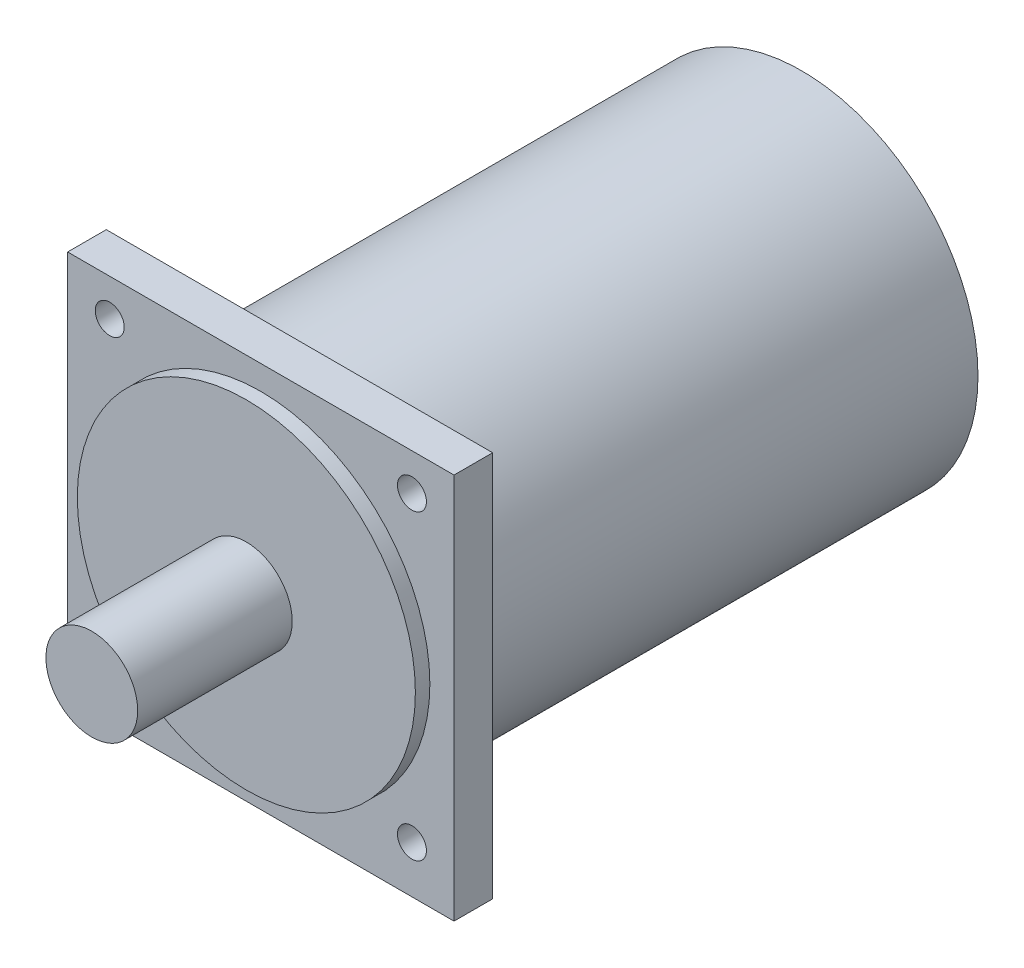
SolidWorks part; units mm, degrees
ref_plane "前视" through (0, 0, 0) normal (0, 0, 1) x (1, 0, 0)
ref_plane "上视" through (0, 0, 0) normal (0, 1, 0) x (1, 0, 0)
ref_plane "右视" through (0, 0, 0) normal (1, 0, 0) x (0, 0, -1)
sketch "草图1" plane through (0, 0, 0) normal (0, 0, 1) x (1, 0, 0)
  line L1 (0, 0) -> (80, 0)
  line L2 (0, 0) -> (0, 80)
  line L3 (0, 80) -> (80, 80)
  line L4 (80, 0) -> (80, 80)
  dimension "D1" = 80
  dimension "D2" = 80
extrude "拉伸1" add sketch "草图1" along normal blind 8
sketch "草图2" plane through (0, 0, 8) normal (0, 0, 1) x (1, 0, 0)
  line L0 (0, 40) -> (80, 40) construction
  line L1 (0, 80) -> (0, 0) construction
  line L2 (80, 0) -> (80, 80) construction
  circle A0 centre (40, 40) radius 35
  dimension "D1" = 70
extrude "拉伸2" add sketch "草图2" along normal blind 3
sketch "草图3" plane through (0, 0, 11) normal (0, 0, 1) x (1, 0, 0)
  circle A0 centre (40, 40) radius 9.5
  circle A1 centre (40, 40) radius 35 construction
  dimension "D1" = 19
extrude "拉伸3" add sketch "草图3" along normal blind 32
sketch "草图4" plane through (0, 0, 0) normal (0, 0, -1) x (-1, 0, 0)
  line L0 (-80, 40) -> (0, 40) construction
  line L1 (-80, 0) -> (-80, 80) construction
  line L2 (0, 80) -> (0, 0) construction
  circle A0 centre (-40, 40) radius 36.4925
extrude "拉伸4" add sketch "草图4" along normal blind 106
sketch "草图5" plane through (0, 0, 8) normal (0, 0, 1) x (1, 0, 0)
  line L0 (40, 82.1163) -> (40, 0) construction
  line L1 (0, 0) -> (80, 0) construction
  line L2 (0, 40) -> (80, 40) construction
  line L3 (0, 80) -> (0, 0) construction
  line L4 (80, 0) -> (80, 80) construction
  line L5 (8.7137, 72.3445) -> (40, 41.0582) construction
  circle A0 centre (8.7137, 72.3445) radius 3
  circle A1 centre (40, 40) radius 9.5 construction
  circle A2 centre (71.2863, 72.3445) radius 3
  circle A3 centre (71.2863, 9.7718) radius 3
  circle A4 centre (8.7137, 9.7718) radius 3
  dimension "D4" = 6
  dimension "D1" = 45
  dimension "D2" = 45
  dimension "D3" = 4
extrude "切除-拉伸1" cut sketch "草图5" against normal up to next
chamfer "倒角1" distance 2 distance2 4 1 edges at (3.5075, 40, -106)
